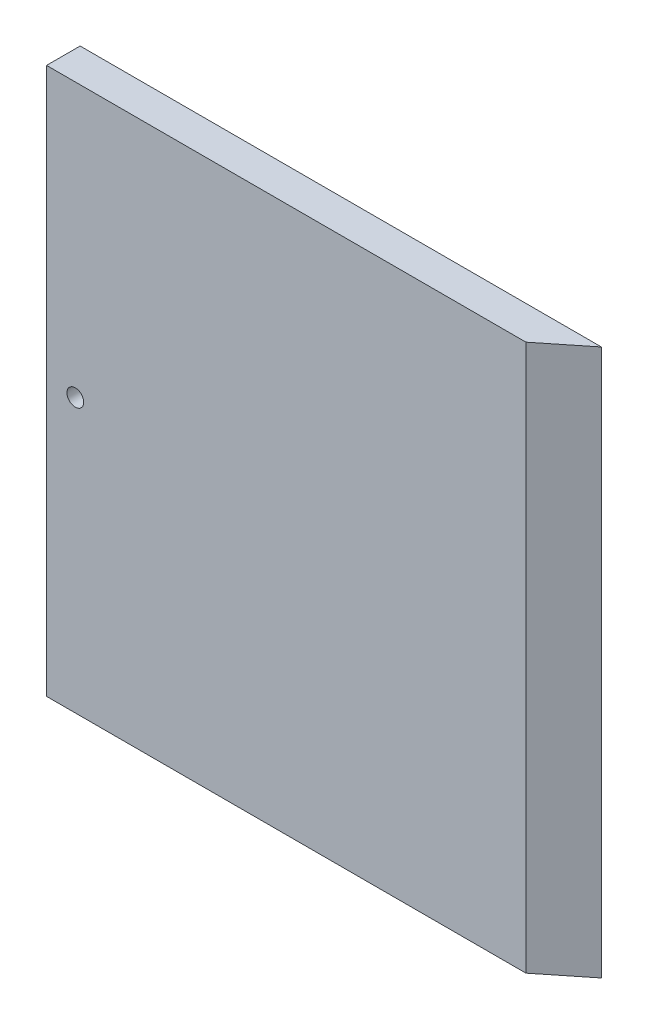
SolidWorks part; units mm, degrees
material "普通碳钢"
ref_plane "Front Plane" through (0, 0, 0) normal (0, 0, 1) x (1, 0, 0)
ref_plane "Top Plane" through (0, 0, 0) normal (0, 1, 0) x (1, 0, 0)
ref_plane "Right Plane" through (0, 0, 0) normal (1, 0, 0) x (0, 0, -1)
sketch "Sketch1" plane through (0, 0, 0) normal (0, 0, 1) x (1, 0, 0)
  line L1 (0, 570) -> (1000, 570)
  line L2 (0, 570) -> (0, 0)
  line L3 (0, 0) -> (1000, 0)
  line L4 (1000, 570) -> (1000, 0)
  dimension "D1" = 570
  dimension "D2" = 1000
extrude "Boss-Extrude1" add sketch "Sketch1" along normal blind 35 contours L2 L3 L4 L1
hole_wizard "M20 Tapped Hole1" positions "3DSketch1" profile "Sketch2" tap size "M20" standard "GB" end condition through all
sketch3d "3DSketch1"
  line L0 (0, 285, 35) -> (1000, 285, 35) construction
  line L1 (0, 570, 35) -> (0, 0, 35) construction
  line L2 (1000, 570, 35) -> (1000, 0, 35) construction
  point P0 (30, 285, 35)
  dimension "D1" = 30
sketch "Sketch2" plane through (30, 285, 35) normal (1, 0, 0) x (0, -1, 0)
  line L0 (0, 0) -> (0, 35)
  line L1 (0, 35) -> (8.75, 35)
  line L2 (8.75, 35) -> (8.75, 0)
  line L5 (8.75, 0) -> (0, 0)
  line L11 (0, -6.35) -> (0, 107.95) construction
  dimension "通孔螺纹孔钻头直径" = 17.5
  dimension "通孔螺纹孔钻头深度" = 35
cosmetic thread "Tapped hole thread 1" parameters "D2"=20
sketch "Sketch3" plane through (0, 0, 35) normal (0, 0, 1) x (1, 0, 0)
  line L0 (500, 570) -> (1000, 570)
  line L1 (0, 570) -> (1000, 570) construction
  line L2 (1000, 570) -> (1000, 270)
  line L3 (1000, 570) -> (1000, 0) construction
  line L4 (1000, 270) -> (500, 570)
  dimension "D1" = 500
  dimension "D2" = 300
sketch "Sketch4" plane through (0, 0, 0) normal (0, -1, 0) x (1, 0, 0)
  line L0 (500, 35) -> (1000, 35)
  line L1 (0, 35) -> (1000, 35) construction
  line L2 (1000, 35) -> (1000, 0) construction
  line L3 (1000, 35) -> (1000, -365)
  line L4 (1000, -365) -> (500, 35)
  dimension "D1" = 500
  dimension "D2" = 400
extrude "Cut-Extrude2" cut sketch "Sketch4" against normal through all
